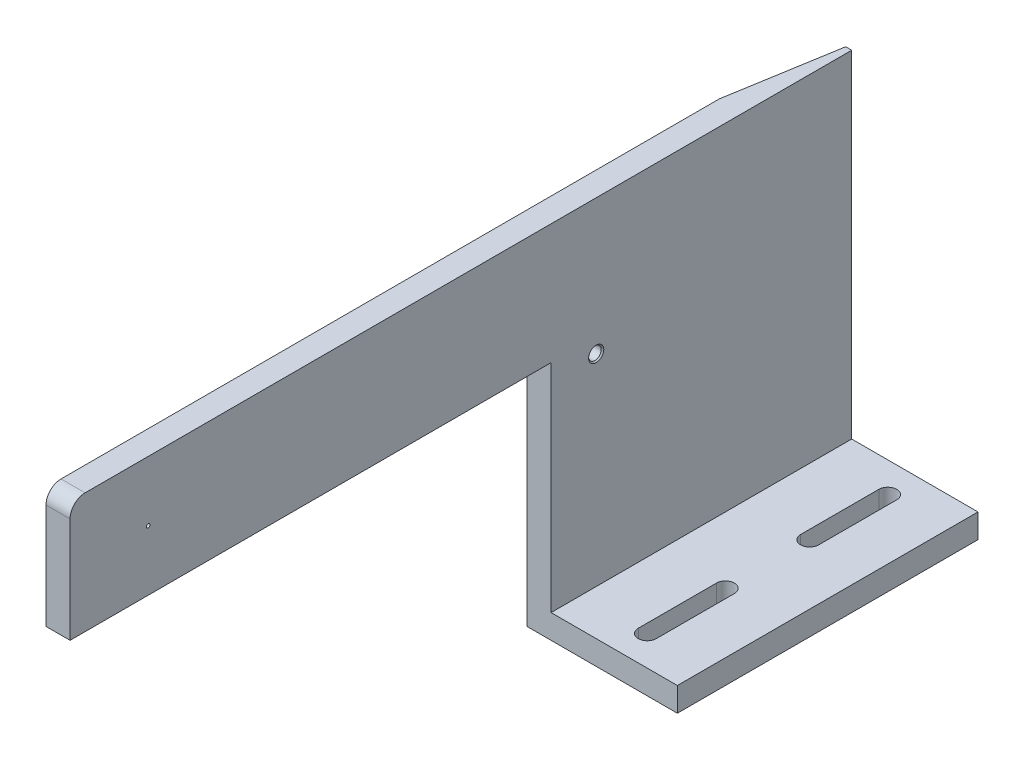
SolidWorks part; units mm, degrees
ref_plane "Front Plane" through (0, 0, 0) normal (0, 0, 1) x (1, 0, 0)
ref_plane "Top Plane" through (0, 0, 0) normal (0, 1, 0) x (1, 0, 0)
ref_plane "Right Plane" through (0, 0, 0) normal (1, 0, 0) x (0, 0, -1)
sketch "Sketch1" plane through (0, 0, 0) normal (0, 0, 1) x (1, 0, 0)
  line L0 (0, 0) -> (0, 120)
  line L1 (0, 0) -> (50, 0)
  line L2 (8, 8) -> (50, 8)
  line L3 (8, 8) -> (8, 120)
  line L4 (50, 8) -> (50, 0)
  line L5 (8, 120) -> (0, 120)
  dimension "D1" = 120
  dimension "D2" = 50
  dimension "D3" = 8
extrude "Boss-Extrude1" add sketch "Sketch1" along normal blind 260
sketch "Sketch2" plane through (50, 0, 0) normal (1, 0, 0) x (0, 0, -1)
  line L0 (-260, 0) -> (0, 0) construction
  line L1 (-100, 0) -> (-260, 0)
  line L2 (-100, 0) -> (-100, 80)
  line L3 (-100, 80) -> (-260, 80)
  line L4 (-260, 0) -> (-260, 80)
  line L5 (0, 8) -> (0, 120) construction
  dimension "D1" = 80
  dimension "D2" = 160
  dimension "D3" = 100
extrude "Cut-Extrude1" cut sketch "Sketch2" against normal through all
sketch "Sketch3" plane through (0, 8, 0) normal (0, 1, 0) x (1, 0, 0)
  line L0 (30, -90) -> (30, -64) construction
  line L1 (27, -90) -> (27, -64)
  line L2 (33, -90) -> (33, -64)
  line L3 (30, -36) -> (30, -10) construction
  line L4 (27, -36) -> (27, -10)
  line L5 (33, -36) -> (33, -10)
  line L6 (50, -100) -> (50, 0) construction
  line L7 (8, -100) -> (50, -100) construction
  line L8 (50, 0) -> (8, 0) construction
  arc A0 (27, -90) -> (33, -90) centre (30, -90) ccw
  arc A1 (33, -64) -> (27, -64) centre (30, -64) ccw
  arc A2 (27, -36) -> (33, -36) centre (30, -36) ccw
  arc A3 (33, -10) -> (27, -10) centre (30, -10) ccw
  point P2 (30, -77)
  point P7 (30, -23)
  dimension "D4" = 26
  dimension "D5" = 26
  dimension "D6" = 10
  dimension "D7" = 10
  dimension "D1" = 6
  dimension "D2" = 6
  dimension "D3" = 20
extrude "Cut-Extrude2" cut sketch "Sketch3" against normal blind 220
sketch "Sketch4" plane through (0, 120, 0) normal (0, 1, 0) x (1, 0, 0)
  line L0 (6, 0) -> (0, -36)
  line L1 (8, 0) -> (0, 0) construction
  line L2 (0, -260) -> (0, 0) construction
  line L3 (0, -36) -> (0, 0)
  line L4 (0, 0) -> (6, 0)
  dimension "D1" = 36
  dimension "D2" = 6
extrude "Cut-Extrude3" cut sketch "Sketch4" against normal through all
hole_wizard "M5 Tapped Hole1" positions "3DSketch1" profile "Sketch5" tap size "M5" standard "GB"
sketch3d "3DSketch1"
  line L0 (8, 80, 100) -> (8, 8, 100) construction
  line L1 (8, 80, 260) -> (8, 80, 100) construction
  point P0 (8, 75, 85)
  dimension "D1" = 15
  dimension "D2" = 5
sketch "Sketch5" plane through (8, 75, 85) normal (0, 1, 0) x (0, 0, -1)
  line L0 (0, 0) -> (0, 7.2618)
  line L1 (0, 7.2618) -> (2.1, 6)
  line L2 (2.1, 6) -> (2.1, 0.425)
  line L3 (2.1, 0.425) -> (2.525, 0)
  line L5 (2.525, 0) -> (0, 0)
  line L6 (-2.1, 0.425) -> (-2.525, 0) construction
  line L10 (0, 7.2618) -> (-2.1, 6) construction
  line L11 (0, -6.35) -> (0, 107.95) construction
  dimension "螺纹孔钻头直径" = 4.2
  dimension "螺纹孔钻头深度" = 6
  dimension "近端锥形沉头孔直径" = 5.05
  dimension "近端锥形沉头孔角度" = 90
  dimension "导头角度" = 118
cosmetic thread "Hole Thread Line1" parameters "D1"=5, "D2"=5
fillet "Fillet1" radius 5 1 edges at (4, 120, 260)
sketch "Sketch6" plane through (8, 0, 0) normal (1, 0, 0) x (0, 0, -1)
  line L0 (-234, 120) -> (-234, 80) construction
  line L1 (-255, 120) -> (0, 120) construction
  line L2 (-260, 80) -> (-100, 80) construction
  line L3 (-260, 80) -> (-260, 115) construction
  circle A0 centre (-234, 100) radius 0.6
  dimension "D2" = 1.2
  dimension "D1" = 26
extrude "Cut-Extrude4" cut sketch "Sketch6" against normal through all
